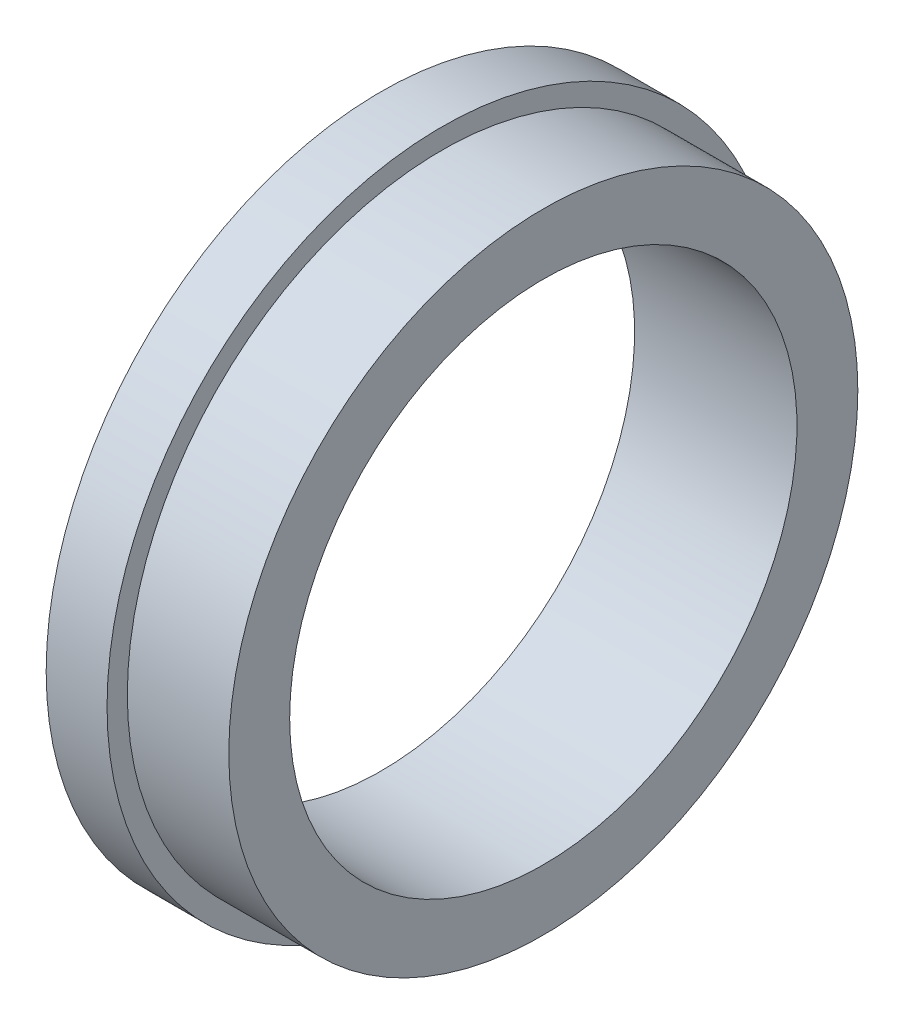
SolidWorks part; units mm, degrees
ref_plane "Front" through (0, 0, 0) normal (0, 0, 1) x (1, 0, 0)
ref_plane "Top" through (0, 0, 0) normal (0, 1, 0) x (1, 0, 0)
ref_plane "Right" through (0, 0, 0) normal (1, 0, 0) x (0, 0, -1)
sketch "Sketch1" plane through (0, 0, 0) normal (0, 0, 1) x (1, 0, 0)
  line L0 (0, 25) -> (16, 25)
  line L1 (16, 25) -> (16, 31)
  line L2 (16, 31) -> (6, 31)
  line L3 (6, 31) -> (6, 33)
  line L4 (6, 33) -> (0, 33)
  line L5 (0, 33) -> (0, 25)
  line L6 (0, 0) -> (76.7648, 0) construction
  dimension "D1" = 6
  dimension "D2" = 2
  dimension "D3" = 16
  dimension "D4" = 8
  dimension "D5" = 25
revolve "Revolve1" add sketch "Sketch1" angle 360 about L6
